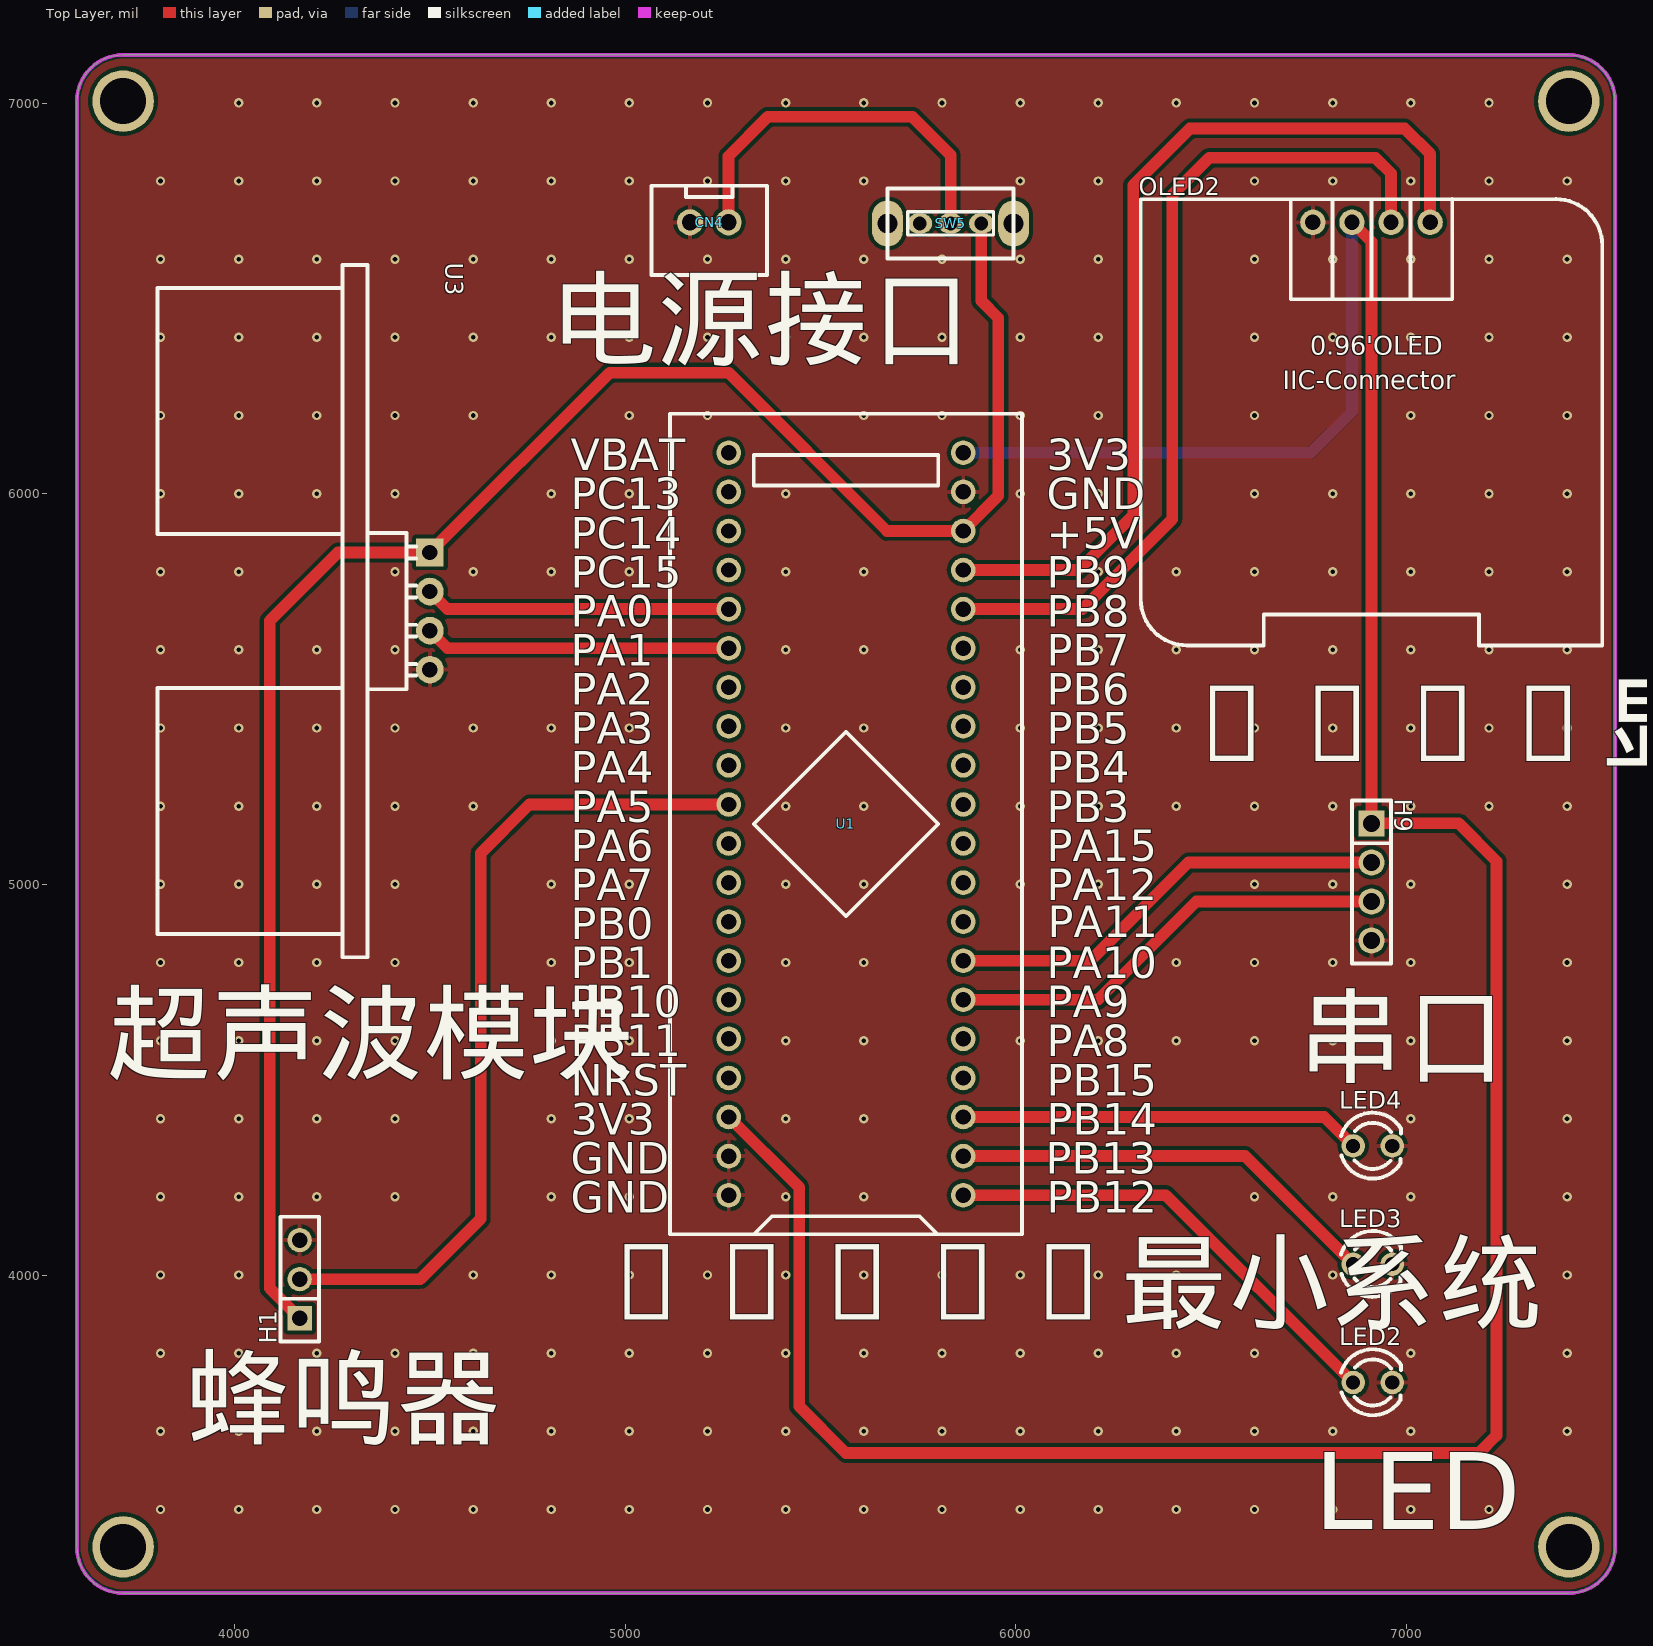
[diagram p0: Top Layer view]
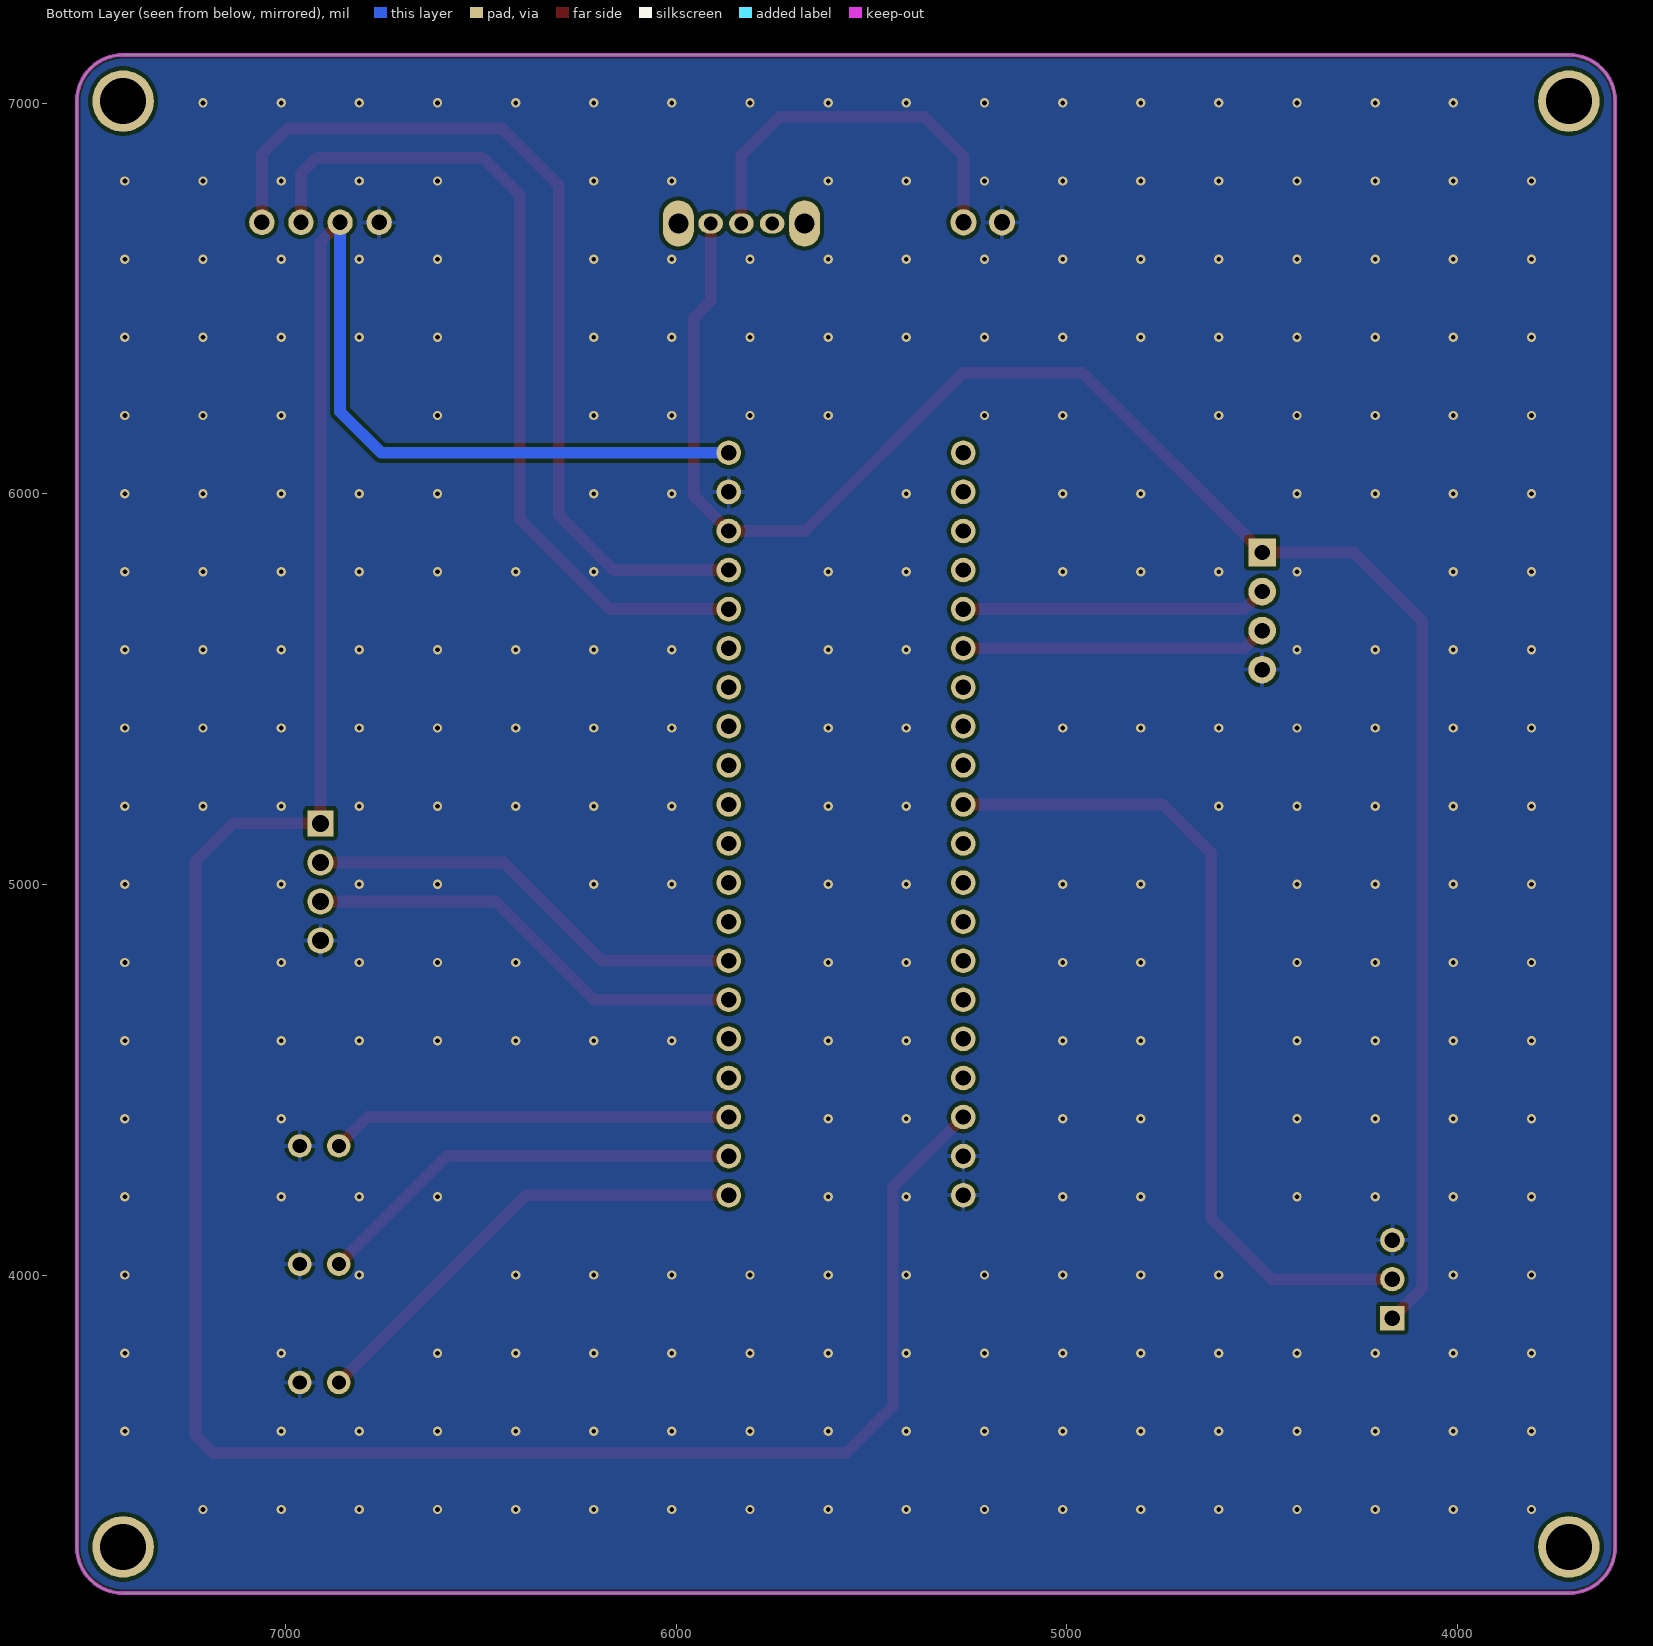
[diagram p1: Bottom Layer view, seen from below]
# Altium PCB MISC51194.pcbdoc
Units mil, origin at the board's own origin, x right, y up, seen from the top; angles counter-clockwise.
Board outline 3937.01 x 3937.01 mil, 2 copper layers (Top Layer, Bottom Layer), stack 62.206 mil thick; 10 components, 38 nets, 72 pads, 291 vias.

## Layer stack, top to bottom
Top Solder Mask Layer: solder mask 0.394, Dk 3.3
Top Layer: signal copper 1.379
Dielectric1: surface 59.449, FR4, Dk 4.5
Bottom Layer: signal copper 1.378
Bottom Solder Mask Layer: solder mask 0.394, Dk 3.3

## Board outline
3714.61,7123.5 ccw(c3714.61,7005.39) 3596.5,7005.39 3596.5,3304.61 ccw(c3714.61,3304.61) 3714.61,3186.5 7415.39,3186.5 ccw(c7415.39,3304.61) 7533.5,3304.61 7533.5,7005.39 ccw(c7415.39,7005.39) 7415.39,7123.5 3714.61,7123.5

## Design rules (kind name [scope] priority, off if disabled: settings)
BoardOutlineClearance copperThickness2oz_1 [All] p2 off: genericclearance=7.99 ignorepadtopadclearanceinfootprint=FALSE except(0: Arc-SplitContinuation Track-SplitContinuation SMDPad-SplitContinuation THPad-SplitContinuation Via-SplitContinuation Fill-SplitContinuation Region-SplitContinuation Poly-SplitContinuation Text-SplitContinuation Hole-SplitContinuation; 5.98: Arc-CutoutEdge Track-CutoutEdge SMDPad-CutoutEdge THPad-CutoutEdge Via-CutoutEdge Text-CutoutEdge; 6.9: Hole-OutlineEdge Hole-CutoutEdge; 10: Poly-OutlineEdge Poly-CutoutEdge; 11.81: Arc-OutlineEdge Track-OutlineEdge SMDPad-OutlineEdge THPad-OutlineEdge Via-OutlineEdge Fill-OutlineEdge Region-OutlineEdge Text-OutlineEdge Fill-CutoutEdge Region-CutoutEdge)
BoardOutlineClearance Plane_innerPlane_1 [All] p4 off: genericclearance=4.02 ignorepadtopadclearanceinfootprint=FALSE except(0: Arc-SplitContinuation Track-SplitContinuation SMDPad-SplitContinuation THPad-SplitContinuation Via-SplitContinuation Fill-SplitContinuation Region-SplitContinuation Poly-SplitContinuation Text-SplitContinuation Hole-SplitContinuation; 5.98: Arc-CutoutEdge Track-CutoutEdge SMDPad-CutoutEdge THPad-CutoutEdge Via-CutoutEdge Text-CutoutEdge; 6.9: Hole-OutlineEdge Hole-CutoutEdge; 10: Poly-OutlineEdge Poly-CutoutEdge; 11.81: Arc-OutlineEdge Track-OutlineEdge SMDPad-OutlineEdge THPad-OutlineEdge Via-OutlineEdge Fill-OutlineEdge Region-OutlineEdge Text-OutlineEdge Fill-CutoutEdge Region-CutoutEdge)
BoardOutlineClearance Copper_copperRegion_1 [All] p6 off: genericclearance=4.02 ignorepadtopadclearanceinfootprint=FALSE except(0: Arc-SplitContinuation Track-SplitContinuation SMDPad-SplitContinuation THPad-SplitContinuation Via-SplitContinuation Fill-SplitContinuation Region-SplitContinuation Poly-SplitContinuation Text-SplitContinuation Hole-SplitContinuation; 5.98: Arc-CutoutEdge Track-CutoutEdge SMDPad-CutoutEdge THPad-CutoutEdge Via-CutoutEdge Text-CutoutEdge; 6.9: Hole-OutlineEdge Hole-CutoutEdge; 10: Poly-OutlineEdge Poly-CutoutEdge; 11.81: Arc-OutlineEdge Track-OutlineEdge SMDPad-OutlineEdge THPad-OutlineEdge Via-OutlineEdge Fill-OutlineEdge Region-OutlineEdge Text-OutlineEdge Fill-CutoutEdge Region-CutoutEdge)
BoardOutlineClearance Copper_copperRegion_copperThickness1oz_1 [All] p8 off: genericclearance=4.02 ignorepadtopadclearanceinfootprint=FALSE except(0: Arc-SplitContinuation Track-SplitContinuation SMDPad-SplitContinuation THPad-SplitContinuation Via-SplitContinuation Fill-SplitContinuation Region-SplitContinuation Poly-SplitContinuation Text-SplitContinuation Hole-SplitContinuation; 5.98: Arc-CutoutEdge Track-CutoutEdge SMDPad-CutoutEdge THPad-CutoutEdge Via-CutoutEdge Text-CutoutEdge; 6.9: Hole-OutlineEdge Hole-CutoutEdge; 10: Poly-OutlineEdge Poly-CutoutEdge; 11.81: Arc-OutlineEdge Track-OutlineEdge SMDPad-OutlineEdge THPad-OutlineEdge Via-OutlineEdge Fill-OutlineEdge Region-OutlineEdge Text-OutlineEdge Fill-CutoutEdge Region-CutoutEdge)
BoardOutlineClearance Copper_copperRegion_Copper_copperRegion_1 [All] p10 off: genericclearance=4.02 ignorepadtopadclearanceinfootprint=FALSE except(0: Arc-SplitContinuation Track-SplitContinuation SMDPad-SplitContinuation THPad-SplitContinuation Via-SplitContinuation Fill-SplitContinuation Region-SplitContinuation Poly-SplitContinuation Text-SplitContinuation Hole-SplitContinuation; 5.98: Arc-CutoutEdge Track-CutoutEdge SMDPad-CutoutEdge THPad-CutoutEdge Via-CutoutEdge Text-CutoutEdge; 6.9: Hole-OutlineEdge Hole-CutoutEdge; 10: Poly-OutlineEdge Poly-CutoutEdge; 11.81: Arc-OutlineEdge Track-OutlineEdge SMDPad-OutlineEdge THPad-OutlineEdge Via-OutlineEdge Fill-OutlineEdge Region-OutlineEdge Text-OutlineEdge Fill-CutoutEdge Region-CutoutEdge)
BoardOutlineClearance copperThickness1oz_1 [All] p12: genericclearance=4.02 ignorepadtopadclearanceinfootprint=FALSE except(0: Arc-SplitContinuation Track-SplitContinuation SMDPad-SplitContinuation THPad-SplitContinuation Via-SplitContinuation Fill-SplitContinuation Region-SplitContinuation Poly-SplitContinuation Text-SplitContinuation Hole-SplitContinuation; 5.98: Arc-CutoutEdge Track-CutoutEdge SMDPad-CutoutEdge THPad-CutoutEdge Via-CutoutEdge Text-CutoutEdge; 6.9: Hole-OutlineEdge Hole-CutoutEdge; 10: Poly-OutlineEdge Poly-CutoutEdge; 11.81: Arc-OutlineEdge Track-OutlineEdge SMDPad-OutlineEdge THPad-OutlineEdge Via-OutlineEdge Fill-OutlineEdge Region-OutlineEdge Text-OutlineEdge Fill-CutoutEdge Region-CutoutEdge)
Clearance copperThickness2oz [All] p1 off: gap=7.99 ignorepadtopadclearanceinfootprint=FALSE except(5.98: SMDPad-Track SMDPad-SMDPad THPad-Track SMDPad-THPad THPad-THPad Track-Via SMDPad-Via THPad-Via Via-Via Fill-SMDPad Region-SMDPad Fill-THPad Region-THPad Fill-Via Region-Via Fill-Fill Fill-Region Region-Region Arc-Track Arc-SMDPad Arc-THPad Arc-Via Fill-Arc Region-Arc Arc-Arc Text-Track SMDPad-Text Text-THPad Text-Via Fill-Text Region-Text Arc-Text Text-Text; 6.9: Hole-Track Hole-SMDPad Hole-THPad Hole-Via Fill-Hole Region-Hole Hole-Arc Hole-Text; 10: Poly-Track Poly-SMDPad Poly-THPad Poly-Via Poly-Fill Poly-Region Poly-Poly Poly-Arc Poly-Text Poly-Hole; 11.81: Fill-Track Region-Track)
Clearance Plane_innerPlane [All] p3 off: gap=4.02 ignorepadtopadclearanceinfootprint=FALSE except(5.98: SMDPad-Track SMDPad-SMDPad THPad-Track SMDPad-THPad THPad-THPad Track-Via SMDPad-Via THPad-Via Via-Via Fill-SMDPad Region-SMDPad Fill-THPad Region-THPad Fill-Via Region-Via Fill-Fill Fill-Region Region-Region Arc-Track Arc-SMDPad Arc-THPad Arc-Via Fill-Arc Region-Arc Arc-Arc Text-Track SMDPad-Text Text-THPad Text-Via Fill-Text Region-Text Arc-Text Text-Text; 6.9: Hole-Track Hole-SMDPad Hole-THPad Hole-Via Fill-Hole Region-Hole Hole-Arc Hole-Text; 10: Poly-Track Poly-SMDPad Poly-THPad Poly-Via Poly-Fill Poly-Region Poly-Poly Poly-Arc Poly-Text Poly-Hole; 11.81: Fill-Track Region-Track)
Clearance Copper_copperRegion [All] p5 off: gap=4.02 ignorepadtopadclearanceinfootprint=FALSE except(5.98: SMDPad-Track SMDPad-SMDPad THPad-Track SMDPad-THPad THPad-THPad Track-Via SMDPad-Via THPad-Via Via-Via Fill-SMDPad Region-SMDPad Fill-THPad Region-THPad Fill-Via Region-Via Fill-Fill Fill-Region Region-Region Arc-Track Arc-SMDPad Arc-THPad Arc-Via Fill-Arc Region-Arc Arc-Arc Text-Track SMDPad-Text Text-THPad Text-Via Fill-Text Region-Text Arc-Text Text-Text; 6.9: Hole-Track Hole-SMDPad Hole-THPad Hole-Via Fill-Hole Region-Hole Hole-Arc Hole-Text; 10: Poly-Track Poly-SMDPad Poly-THPad Poly-Via Poly-Fill Poly-Region Poly-Poly Poly-Arc Poly-Text Poly-Hole; 11.81: Fill-Track Region-Track)
Clearance Copper_copperRegion_copperThickness1oz [All] p7 off: gap=4.02 ignorepadtopadclearanceinfootprint=FALSE except(5.98: SMDPad-Track SMDPad-SMDPad THPad-Track SMDPad-THPad THPad-THPad Track-Via SMDPad-Via THPad-Via Via-Via Fill-SMDPad Region-SMDPad Fill-THPad Region-THPad Fill-Via Region-Via Fill-Fill Fill-Region Region-Region Arc-Track Arc-SMDPad Arc-THPad Arc-Via Fill-Arc Region-Arc Arc-Arc Text-Track SMDPad-Text Text-THPad Text-Via Fill-Text Region-Text Arc-Text Text-Text; 6.9: Hole-Track Hole-SMDPad Hole-THPad Hole-Via Fill-Hole Region-Hole Hole-Arc Hole-Text; 10: Poly-Track Poly-SMDPad Poly-THPad Poly-Via Poly-Fill Poly-Region Poly-Poly Poly-Arc Poly-Text Poly-Hole; 11.81: Fill-Track Region-Track)
Clearance Copper_copperRegion_Copper_copperRegion [All] p9 off: gap=4.02 ignorepadtopadclearanceinfootprint=FALSE except(5.98: SMDPad-Track SMDPad-SMDPad THPad-Track SMDPad-THPad THPad-THPad Track-Via SMDPad-Via THPad-Via Via-Via Fill-SMDPad Region-SMDPad Fill-THPad Region-THPad Fill-Via Region-Via Fill-Fill Fill-Region Region-Region Arc-Track Arc-SMDPad Arc-THPad Arc-Via Fill-Arc Region-Arc Arc-Arc Text-Track SMDPad-Text Text-THPad Text-Via Fill-Text Region-Text Arc-Text Text-Text; 6.9: Hole-Track Hole-SMDPad Hole-THPad Hole-Via Fill-Hole Region-Hole Hole-Arc Hole-Text; 10: Poly-Track Poly-SMDPad Poly-THPad Poly-Via Poly-Fill Poly-Region Poly-Poly Poly-Arc Poly-Text Poly-Hole; 11.81: Fill-Track Region-Track)
Clearance copperThickness1oz [All] p11: gap=4.02 ignorepadtopadclearanceinfootprint=FALSE except(5.98: SMDPad-Track SMDPad-SMDPad THPad-Track SMDPad-THPad THPad-THPad Track-Via SMDPad-Via THPad-Via Via-Via Fill-SMDPad Region-SMDPad Fill-THPad Region-THPad Fill-Via Region-Via Fill-Fill Fill-Region Region-Region Arc-Track Arc-SMDPad Arc-THPad Arc-Via Fill-Arc Region-Arc Arc-Arc Text-Track SMDPad-Text Text-THPad Text-Via Fill-Text Region-Text Arc-Text Text-Text; 6.9: Hole-Track Hole-SMDPad Hole-THPad Hole-Via Fill-Hole Region-Hole Hole-Arc Hole-Text; 10: Poly-Track Poly-SMDPad Poly-THPad Poly-Via Poly-Fill Poly-Region Poly-Poly Poly-Arc Poly-Text Poly-Hole; 11.81: Fill-Track Region-Track)
DiffPairsRouting differentialPair [All] p1: maxlimit=6 minlimit=6 mostfreqgap=6 toplayer_minwidth=5 toplayer_prefwidth=10 toplayer_maxwidth=100 toplayer_mingap=6 toplayer_prefgap=6 toplayer_maxgap=6 bottomlayer_minwidth=5 bottomlayer_prefwidth=10 bottomlayer_maxwidth=100 bottomlayer_mingap=6 bottomlayer_prefgap=6 bottomlayer_maxgap=6 maxuncoupledlength=10
HoleToHoleClearance otherClearance [All] p1: gap=11.81 allowstackedmicrovias=TRUE
Length netLength [All] p1: minlimit=0 maxlimit=0
PasteMaskExpansion pasteMaskExpansion [All] p1: expansion=0
PlaneConnect innerPlane [All] p1: planeconnectstyle=Relief reliefexpansion=20 reliefentries=4 reliefconductorwidth=10 reliefairgap=10
PolygonConnect copperRegion_copperThickness1oz [All] p1 off: connectstyle=Relief reliefconductorwidth=10 reliefentries=4 polygonreliefangle="90 Angle" airgapwidth=10 via.connectstyle=Relief via.reliefconductorwidth=10 via.reliefentries=4 via.polygonreliefangle="90 Angle" via.airgapwidth=10
PolygonConnect copperRegion_Copper_copperRegion [All] p2 off: connectstyle=Relief reliefconductorwidth=10 reliefentries=4 polygonreliefangle="90 Angle" airgapwidth=10 via.connectstyle=Relief via.reliefconductorwidth=10 via.reliefentries=4 via.polygonreliefangle="90 Angle" via.airgapwidth=10
PolygonConnect copperRegion [All] p3: connectstyle=Relief reliefconductorwidth=10 reliefentries=4 polygonreliefangle="90 Angle" airgapwidth=10 via.connectstyle=Relief via.reliefconductorwidth=10 via.reliefentries=4 via.polygonreliefangle="90 Angle" via.airgapwidth=10
RoutingVias viaSize [All] p1: holewidth=12.01 width=24.02 viastyle="Through Hole" minholewidth=11.81 minwidth=19.68 maxholewidth=248.03 maxwidth=393.7
SolderMaskExpansion solderMaskExpansion [IsVia] p1: expansion=-1000 istentingtop=TRUE
SolderMaskExpansion solderMaskExpansion [All] p2: expansion=2 istentingtop=FALSE
Width copperThickness2oz_2 [All] p1 off: maxlimit=100 minlimit=8 preferedwidth=10
Width copperThickness1oz_2 [All] p2: maxlimit=100 minlimit=5 preferedwidth=10

## Components (designator, comment, footprint, x,y, rotation, side; value= is the part's Value field where it differs from the comment)
CN4 "XH2.54*2P_直插" CONN-TH_2P-P2.50-XH2.54-2P 5215,6695 r0 top
H1 "" HDR-TH_3P-P2.54-V-F 4166.72,3990 r90 top
H9 "" HDR-TH_4P-P2.54-V-F 6910,5006.63 r270 top
LED2 "" LED_TH-3mm 6913.13,3725.6 r0 top
LED3 "" LED_TH-3mm 6913.13,4028.36 r0 top
LED4 "" LED_TH-3mm 6913.13,4331.11 r0 top
OLED2 "" 0.96OLED_4P 6910,6695 r0 top
SW5 "" 拨动开关 5837.9,6692.05 r180 top
U1 "STM32F103C8T6-Card" CONN-TH_L53.3-W22.9_STM32F103C8T6-CARD 5565,5155 r90 top
U3 "HC-SR04" TH_HC-SR04V 4500,5700 r270 top

## Footprints (in the part's own frame and the unit in brackets; to place one, negate y for a bottom-side part, rotate by r counter-clockwise, add the part's x,y. Pads: shape width x height; smd on the part's side, far side on the other; paste and mask are expansions set on the pad)
0.96OLED_4P [mm]
  round 1.65 hole 1 copper offset 0,0: 1(-3.81,-0.001) 2(-1.27,0.002) 3(1.27,0.002) 4(3.81,0.002)
  silkscreen extent -15,-27.5 15,1.5
CONN-TH_2P-P2.50-XH2.54-2P [mm]
  round 1.7 hole 1.05 paste+0 mask+0.05: 1(1.25,0) 2(-1.25,0)
  silkscreen extent -3.75,-3.42 3.75,2.37
CONN-TH_L53.3-W22.9_STM32F103C8T6-CARD [mm]
  round 1.6 hole 1: 1(-24.13,-7.62) 2(-21.59,-7.62) 3(-19.05,-7.62) 4(-16.51,-7.62) 5(-13.97,-7.62) 6(-11.43,-7.62) 7(-8.89,-7.62) 8(-6.35,-7.62) 9(-3.81,-7.62) 10(-1.27,-7.62) 11(1.27,-7.62) 12(3.81,-7.62) 13(6.35,-7.62) 14(8.89,-7.62) 15(11.43,-7.62) 16(13.97,-7.62) 17(16.51,-7.62) 18(19.05,-7.62) 19(21.59,-7.62) 20(24.13,-7.62) 21(24.13,7.62) 22(21.59,7.62) 23(19.05,7.62) 24(16.51,7.62) 25(13.97,7.62) 26(11.43,7.62) 27(8.89,7.62) 28(6.35,7.62) 29(3.81,7.62) 30(1.27,7.62) 31(-1.27,7.62) 32(-3.81,7.62) 33(-6.35,7.62) 34(-8.89,7.62) 35(-11.43,7.62) 36(-13.97,7.62) 37(-16.51,7.62) 38(-19.05,7.62) 39(-21.59,7.62) 40(-24.13,7.62)
  silkscreen extent -26.67,-11.43 26.67,11.43
HDR-TH_3P-P2.54-V-F [mil]
  rect 62x62 hole 40.16: 1(-100,0)
  round 62 hole 40.16: 2(0,0) 3(100,0)
  silkscreen extent -160,-49 160,49
HDR-TH_4P-P2.54-V-F [mm]
  rect 1.7x1.7 hole 1.1: 1(-3.81,0)
  round 1.7 hole 1.1: 2(-1.27,0) 3(1.27,0) 4(3.81,0)
  silkscreen extent -5.29,-1.27 5.29,1.27
LED_TH-3mm [mil]
  round 60 hole 36 paste+0 mask+2: 1(-50,0) 2(50,0)
  silkscreen extent -81,-84 72,85
TH_HC-SR04V [mm]
  rect 1.8x1.8 hole 1.001: 1(-3.81,0)
  round 1.8 hole 1.001: 2(-1.27,0) 3(1.27,0) 4(3.81,0)
  silkscreen extent -22.5,-17.7 22.5,-0.89
拨动开关 [mil]
  oval 63x51.2 hole 35.4 paste+0 mask+2: 1(-73.4,0) 2(5,0) 3(84,0)
  oval 78.7x118.1 hole 51.2 paste+0 mask+2: 4(166.7,0) 5(-156.1,0)
  silkscreen extent -156,-90 167,90

## Free pads (board coordinates)
  round 157.48 hole 118.11: 1(3714.61,7005.39) 1(3714.61,3304.61) 1(7415.39,7005.39) 1(7415.39,3304.61)

## Via types
v1: diameter 24.02, hole 12, Top Layer to Bottom Layer, 291 vias

## Nets (pads, with @x,y where several pads share a name; then routed paths per layer and width w, separated by ;. In a path a pad name is that pad's centre, name@x,y a point inside that pad or via, vN(x,y) a via of type N, cw(c..) or ccw(c..) an arc to the next point about the centre after c; other vN are vias at no path point)
$1N17118: CN4.1 SW5.2 | length 995.2
  Top Layer w30: CN4.1 5264.22,6864.22 5365,6965 5735,6965 5832.9,6867.1 SW5.2
+5V: H1.1 SW5.1 U1.18 U3.1 | length 4865
  Top Layer w30: H1.1 4090,3966.72 4090,5675 4265,5850 U3.1 4960,6310 5265,6310 5670,5905 U1.18 5955,5995 5955,6450 5911.3,6493.7 SW5.1
GND: CN4.2 H1.3 H9.4 LED2.2 LED3.2 LED4.2 OLED2.1 U1.19 U1.39 U1.40 U3.4
  other v1: 3810.6,3400.6 4010.6,3400.6 4210.6,3400.6 4410.6,3400.6 4610.6,3400.6 4810.6,3400.6 5010.6,3400.6 5210.6,3400.6 5410.6,3400.6 5610.6,3400.6 5810.6,3400.6 6010.6,3400.6 6210.6,3400.6 6410.6,3400.6 6610.6,3400.6 6810.6,3400.6 7010.6,3400.6 7210.6,3400.6 3810.6,3600.6 4010.6,3600.6 4210.6,3600.6 4410.6,3600.6 4610.6,3600.6 4810.6,3600.6 5010.6,3600.6 5210.6,3600.6 5410.6,3600.6 5610.6,3600.6 5810.6,3600.6 6010.6,3600.6 6210.6,3600.6 6410.6,3600.6 6610.6,3600.6 6810.6,3600.6 7010.6,3600.6 7410.6,3600.6 3810.6,3800.6 4010.6,3800.6 4210.6,3800.6 4410.6,3800.6 4610.6,3800.6 4810.6,3800.6 5010.6,3800.6 5210.6,3800.6 5410.6,3800.6 5610.6,3800.6 5810.6,3800.6 6010.6,3800.6 6210.6,3800.6 6410.6,3800.6 6610.6,3800.6 7010.6,3800.6 7410.6,3800.6 3810.6,4000.6 4010.6,4000.6 4610.6,4000.6 4810.6,4000.6 5010.6,4000.6 5210.6,4000.6 5410.6,4000.6 5610.6,4000.6 5810.6,4000.6 6010.6,4000.6 6210.6,4000.6 6410.6,4000.6 6810.6,4000.6 7410.6,4000.6 3810.6,4200.6 4010.6,4200.6 4210.6,4200.6 4410.6,4200.6 4810.6,4200.6 5010.6,4200.6 5410.6,4200.6 5610.6,4200.6 6610.6,4200.6 6810.6,4200.6 7010.6,4200.6 7410.6,4200.6 3810.6,4400.6 4010.6,4400.6 4210.6,4400.6 4410.6,4400.6 4810.6,4400.6 5010.6,4400.6 5410.6,4400.6 5610.6,4400.6 7010.6,4400.6 7410.6,4400.6 3810.6,4600.6 4010.6,4600.6 4210.6,4600.6 4410.6,4600.6 4810.6,4600.6 5010.6,4600.6 5410.6,4600.6 5610.6,4600.6 6010.6,4600.6 6210.6,4600.6 6410.6,4600.6 6610.6,4600.6 6810.6,4600.6 7010.6,4600.6 7410.6,4600.6 3810.6,4800.6 4010.6,4800.6 4210.6,4800.6 4410.6,4800.6 4810.6,4800.6 5010.6,4800.6 5410.6,4800.6 5610.6,4800.6 6410.6,4800.6 6610.6,4800.6 6810.6,4800.6 7010.6,4800.6 7410.6,4800.6 3810.6,5000.6 4010.6,5000.6 4210.6,5000.6 4410.6,5000.6 4810.6,5000.6 5010.6,5000.6 5410.6,5000.6 5610.6,5000.6 6010.6,5000.6 6210.6,5000.6 6610.6,5000.6 6810.6,5000.6 7010.6,5000.6 7410.6,5000.6 3810.6,5200.6 4010.6,5200.6 4210.6,5200.6 4410.6,5200.6 4610.6,5200.6 5410.6,5200.6 5610.6,5200.6 6010.6,5200.6 6210.6,5200.6 6410.6,5200.6 6610.6,5200.6 6810.6,5200.6 7010.6,5200.6 7210.6,5200.6 7410.6,5200.6 3810.6,5400.6 4010.6,5400.6 4210.6,5400.6 4410.6,5400.6 4610.6,5400.6 4810.6,5400.6 5010.6,5400.6 5410.6,5400.6 5610.6,5400.6 6010.6,5400.6 6210.6,5400.6 6410.6,5400.6 6610.6,5400.6 6810.6,5400.6 7010.6,5400.6 7210.6,5400.6 7410.6,5400.6 3810.6,5600.6 4010.6,5600.6 4210.6,5600.6 4410.6,5600.6 5410.6,5600.6 5610.6,5600.6 6010.6,5600.6 6210.6,5600.6 6410.6,5600.6 6610.6,5600.6 6810.6,5600.6 7010.6,5600.6 7210.6,5600.6 7410.6,5600.6 3810.6,5800.6 4010.6,5800.6 4410.6,5800.6 4610.6,5800.6 4810.6,5800.6 5010.6,5800.6 5410.6,5800.6 5610.6,5800.6 6210.6,5800.6 6410.6,5800.6 6610.6,5800.6 6810.6,5800.6 7010.6,5800.6 7210.6,5800.6 7410.6,5800.6 3810.6,6000.6 4010.6,6000.6 4210.6,6000.6 4410.6,6000.6 4810.6,6000.6 5010.6,6000.6 5410.6,6000.6 6010.6,6000.6 6210.6,6000.6 6610.6,6000.6 6810.6,6000.6 7010.6,6000.6 7210.6,6000.6 7410.6,6000.6 3810.6,6200.6 4010.6,6200.6 4210.6,6200.6 4410.6,6200.6 4610.6,6200.6 5010.6,6200.6 5210.6,6200.6 5610.6,6200.6 5810.6,6200.6 6010.6,6200.6 6210.6,6200.6 6610.6,6200.6 7010.6,6200.6 7210.6,6200.6 7410.6,6200.6 3810.6,6400.6 4010.6,6400.6 4210.6,6400.6 4410.6,6400.6 4610.6,6400.6 4810.6,6400.6 5010.6,6400.6 5210.6,6400.6 5410.6,6400.6 5610.6,6400.6 5810.6,6400.6 6010.6,6400.6 6210.6,6400.6 6610.6,6400.6 6810.6,6400.6 7010.6,6400.6 7210.6,6400.6 7410.6,6400.6 3810.6,6600.6 4010.6,6600.6 4210.6,6600.6 4410.6,6600.6 4610.6,6600.6 4810.6,6600.6 5010.6,6600.6 5210.6,6600.6 5410.6,6600.6 5610.6,6600.6 5810.6,6600.6 6010.6,6600.6 6210.6,6600.6 6610.6,6600.6 6810.6,6600.6 7010.6,6600.6 7210.6,6600.6 7410.6,6600.6 3810.6,6800.6 4010.6,6800.6 4210.6,6800.6 4410.6,6800.6 4610.6,6800.6 4810.6,6800.6 5010.6,6800.6 5210.6,6800.6 5410.6,6800.6 5610.6,6800.6 6010.6,6800.6 6210.6,6800.6 6610.6,6800.6 6810.6,6800.6 7010.6,6800.6 7210.6,6800.6 7410.6,6800.6 4010.6,7000.6 4210.6,7000.6 4410.6,7000.6 4610.6,7000.6 4810.6,7000.6 5010.6,7000.6 5210.6,7000.6 5410.6,7000.6 5610.6,7000.6 5810.6,7000.6 6010.6,7000.6 6210.6,7000.6 6410.6,7000.6 6610.6,7000.6 6810.6,7000.6 7010.6,7000.6 7210.6,7000.6
NRST: U1.37
PA0: U1.25 U3.2 | length 783.6
  Top Layer w30: U3.2 4545,5705 U1.25
PA1: U1.26 U3.3 | length 783.6
  Top Layer w30: U3.3 4545,5605 U1.26
PA2: U1.27
PA3: U1.28
PA4: U1.29
PA5: H1.2 U1.30 | length 2149.3
  Top Layer w30: H1.2 4475,3990 4630,4145 4630,5080 4755,5205 U1.30
PA6: U1.31
PA7: U1.32
PA8: U1.5
PA9: H9.3 U1.6 | length 1149.2
  Top Layer w30: U1.6 6210,4705 6461.63,4956.63 H9.3
PA10: H9.2 U1.7 | length 1149.2
  Top Layer w30: U1.7 6190,4805 6441.63,5056.63 H9.2
PA11: U1.8
PA12: U1.9
PA15: U1.10
PB0: U1.33
PB1: U1.34
PB3: U1.11
PB4: U1.12
PB5: U1.13
PB6: U1.14
PB7: U1.15
PB8: OLED2.3 U1.16 | length 2201.1
  Top Layer w30: U1.16 6170,5705 6400,5935 6400,6765 6495,6860 6920,6860 6960,6820 OLED2.3@6960,6695.05
PB9: OLED2.4 U1.17 | length 2359.9
  Top Layer w30: U1.17 6160,5805 6300,5945 6300,6790 6445,6935 6995,6935 7060,6870 OLED2.4@7060,6695.05
PB10: U1.35
PB11: U1.36
PB12: LED2.1 U1.1 | length 1196.7
  Top Layer w30: U1.1 6383.73,4205 LED2.1
PB13: LED3.1 U1.2 | length 1112.7
  Top Layer w30: U1.2 6586.48,4305 LED3.1
PB14: LED4.1 U1.3 | length 1028.7
  Top Layer w30: U1.3 6789.23,4405 LED4.1
PB15: U1.4
PC13: U1.22
PC14: U1.23
PC15: U1.24
VBAT: U1.21
VCC: H9.1 OLED2.2 U1.20 U1.38 | length 7580.6
  Top Layer w30: U1.38 5445,4225 5445,3665 5565,3545 7185,3545 7230,3590 7230,5060 7133.37,5156.63 H9.1 6910,6645.05 OLED2.2@6860,6695.05
  Bottom Layer w30: U1.20 6755,6105 6860,6210 OLED2.2@6860,6695.05
pads on no net: SW5.3 SW5.4 SW5.5

## Polygon pours and split planes (outlines as drawn)
GND on Bottom Layer (solid, remove dead copper, pour order 2): 3525,7245 3525,3080 7700,3080 7700,7245
GND on Top Layer (solid, remove dead copper, pour order 2): 3000,7415 3000,3000 7930,3000 7930,7415

## Keep-outs
Board Outline Layer:
  the board outline again, w10

## Silkscreen, mask and mechanical layers (free items; w line width, h text height)
Top Silkscreen Layer:
  text "电源接口" at 4812.87,6351.57 h196.85
  text "VBAT" at 4860.95,6060 h80
  text "3V3" at 6079.16,6060 h80
  text "PC13" at 4860.95,5960 h80
  text "GND" at 6079.16,5960 h80
  text "PC14" at 4860.95,5860 h80
  text "+5V" at 6079.16,5860 h80
  text "PC15" at 4860.95,5760 h80
  text "PB9" at 6079.16,5760 h80
  text "PA0" at 4860.95,5660 h80
  text "PB8" at 6079.16,5660 h80
  text "PA1" at 4860.95,5560 h80
  text "PB7" at 6079.16,5560 h80
  text "PA2" at 4860.95,5460 h80
  text "PB6" at 6079.16,5460 h80
  text "PA3" at 4860.95,5360 h80
  text "PB5" at 6079.16,5360 h80
  text "Oled显示器" at 6418.02,5315.2 h196.85
  text "PA4" at 4860.95,5260 h80
  text "PB4" at 6079.16,5260 h80
  text "PA5" at 4860.95,5160 h80
  text "PB3" at 6079.16,5160 h80
  text "PA6" at 4860.95,5060 h80
  text "PA15" at 6079.16,5060 h80
  text "PA7" at 4860.95,4960 h80
  text "PA12" at 6079.16,4960 h80
  text "PA11" at 6080.95,4865 h80
  text "PB0" at 4860.95,4860 h80
  text "PB1" at 4860.95,4760 h80
  text "PA10" at 6079.16,4760 h80
  text "PB10" at 4860.95,4660 h80
  text "PA9" at 6079.16,4660 h80
  text "PB11" at 4860.95,4560 h80
  text "PA8" at 6079.16,4560 h80
  text "超声波模块" at 3673.55,4525 h196.85
  text "串口" at 6721.2,4515.22 h196.85
  text "NRST" at 4860.95,4460 h80
  text "PB15" at 6079.16,4460 h80
  text "3V3" at 4860.95,4360 h80
  text "PB14" at 6079.16,4360 h80
  text "GND" at 4860.95,4260 h80
  text "PB13" at 6075.95,4260 h80
  text "GND" at 4860.95,4160 h80
  text "PB12" at 6079.16,4160 h80
  text "STM32最小系统" at 4919.45,3886.57 h196.85
  text "蜂鸣器" at 3873.53,3590 h196.85
  text "LED" at 6762.95,3350 h196.85